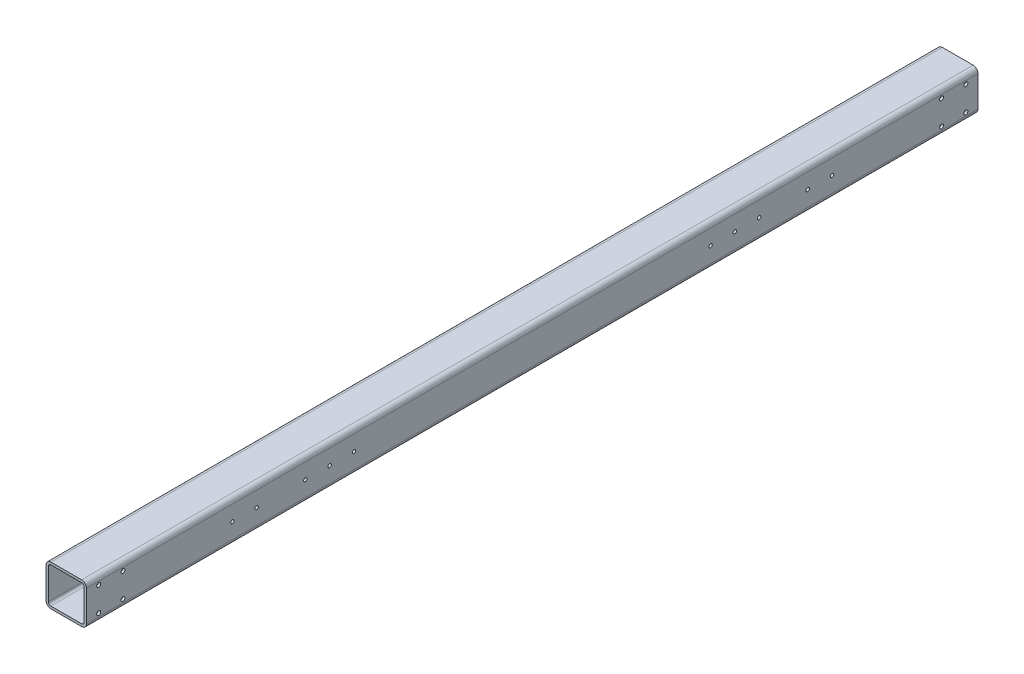
from build123d import *

# Parameters (mm, degrees)
GB_6728_1986_050_X_50_X_3_1_DEPTH = 1100
HOLE_WIZARD_M5_1_D                = 4.2
HOLE_WIZARD_M5_1_DEPTH            = 12.4
HOLE_WIZARD_M5_1_TIP              = 1.2618073
HOLE_WIZARD_M5_2_D                = 4.2
HOLE_WIZARD_M5_2_DEPTH            = 15
HOLE_WIZARD_M5_2_TIP              = 1.2618073
HOLE_WIZARD_M5_3_D                = 4.2
HOLE_WIZARD_M5_3_DEPTH            = 12.4
HOLE_WIZARD_M5_3_TIP              = 1.2618073
HOLE_WIZARD_M6_1_D                = 5
HOLE_WIZARD_M6_1_DEPTH            = 15
HOLE_WIZARD_M6_1_TIP              = 1.502151548


with BuildPart() as part:
    # Sketch1 → Gb／6728-1986方形空心型钢 050 X 50 X 3(1) (new body)
    with BuildSketch(Plane(origin=(0, 0, 0), x_dir=(-1, 0, 0), z_dir=(0, 0, -1))):
        with BuildLine():
            Line((-19, -25), (19, -25))
            ThreePointArc((19, -25), (23.242640687, -23.242640687), (25, -19))
            Line((25, -19), (25, 19))
            ThreePointArc((25, 19), (23.242640687, 23.242640687), (19, 25))
            Line((19, 25), (-19, 25))
            ThreePointArc((-19, 25), (-23.242640687, 23.242640687), (-25, 19))
            Line((-25, 19), (-25, -19))
            ThreePointArc((-25, -19), (-23.242640687, -23.242640687), (-19, -25))
        make_face()
        with BuildLine():
            Line((-19, -22), (19, -22))
            ThreePointArc((19, -22), (21.121320344, -21.121320344), (22, -19))
            Line((22, -19), (22, 19))
            ThreePointArc((22, 19), (21.121320344, 21.121320344), (19, 22))
            Line((19, 22), (-19, 22))
            ThreePointArc((-19, 22), (-21.121320344, 21.121320344), (-22, 19))
            Line((-22, 19), (-22, -19))
            ThreePointArc((-22, -19), (-21.121320344, -21.121320344), (-19, -22))
        make_face(mode=Mode.SUBTRACT)
    extrude(amount=GB_6728_1986_050_X_50_X_3_1_DEPTH)

    # M5 螺纹孔1
    with Locations(Plane(origin=(25, 0, 0), x_dir=(0, 0, -1), z_dir=(1, 0, 0))):
        with Locations((180, 0), (210, 0)):
            Hole(HOLE_WIZARD_M5_1_D / 2, depth=HOLE_WIZARD_M5_1_DEPTH)
            with Locations((0, 0, -(HOLE_WIZARD_M5_1_DEPTH + HOLE_WIZARD_M5_1_TIP / 2))):  # 118° drill point
                Cone(0, HOLE_WIZARD_M5_1_D / 2, HOLE_WIZARD_M5_1_TIP, mode=Mode.SUBTRACT)

    # M5 螺纹孔2
    with Locations(Plane(origin=(25, 0, 0), x_dir=(0, 0, -1), z_dir=(1, 0, 0))):
        with Locations((270, 0), (300, 0), (330, 0)):
            Hole(HOLE_WIZARD_M5_2_D / 2, depth=HOLE_WIZARD_M5_2_DEPTH)
            with Locations((0, 0, -(HOLE_WIZARD_M5_2_DEPTH + HOLE_WIZARD_M5_2_TIP / 2))):  # 118° drill point
                Cone(0, HOLE_WIZARD_M5_2_D / 2, HOLE_WIZARD_M5_2_TIP, mode=Mode.SUBTRACT)

    # M5 螺纹孔3
    with Locations(Plane(origin=(25, 0, 0), x_dir=(0, 0, -1), z_dir=(1, 0, 0))):
        with Locations((920, 0), (890, 0), (830, 0), (800, 0), (770, 0)):
            Hole(HOLE_WIZARD_M5_3_D / 2, depth=HOLE_WIZARD_M5_3_DEPTH)
            with Locations((0, 0, -(HOLE_WIZARD_M5_3_DEPTH + HOLE_WIZARD_M5_3_TIP / 2))):  # 118° drill point
                Cone(0, HOLE_WIZARD_M5_3_D / 2, HOLE_WIZARD_M5_3_TIP, mode=Mode.SUBTRACT)

    # M6 螺纹孔1
    with Locations(Plane(origin=(25, 0, 0), x_dir=(0, 0, -1), z_dir=(1, 0, 0))):
        with Locations((15, 15), (45, 15), (15, -15), (45, -15), (1055, 15), (1085, 15), (1055, -15), (1085, -15)):
            Hole(HOLE_WIZARD_M6_1_D / 2, depth=HOLE_WIZARD_M6_1_DEPTH)
            with Locations((0, 0, -(HOLE_WIZARD_M6_1_DEPTH + HOLE_WIZARD_M6_1_TIP / 2))):  # 118° drill point
                Cone(0, HOLE_WIZARD_M6_1_D / 2, HOLE_WIZARD_M6_1_TIP, mode=Mode.SUBTRACT)


solid = part.part
